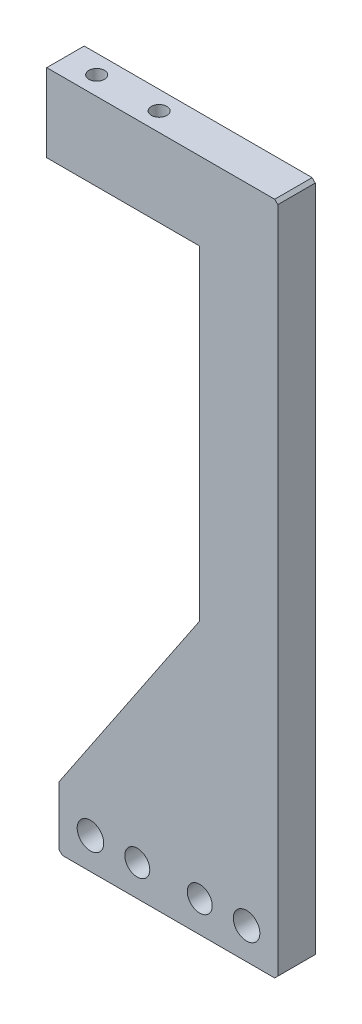
SolidWorks part; units mm, degrees
material "AISI 1045 钢，冷拔"
ref_plane "前视基准面" through (0, 0, 0) normal (0, 0, 1) x (1, 0, 0)
ref_plane "上视基准面" through (0, 0, 0) normal (0, 1, 0) x (1, 0, 0)
ref_plane "右视基准面" through (0, 0, 0) normal (1, 0, 0) x (0, 0, -1)
sketch "草图1" plane through (0, 0, 0) normal (0, 0, 1) x (1, 0, 0)
  line L0 (74.8691, -20) -> (4.8691, -20)
  line L1 (4.8691, -20) -> (4.8691, 0)
  line L3 (4.8691, 0) -> (49.8691, 67.0298)
  line L5 (49.8691, 67.0298) -> (49.8691, 171)
  line L6 (49.8691, 171) -> (0.8691, 171)
  line L7 (0.8691, 171) -> (0.8691, 196)
  line L8 (0.8691, 196) -> (74.8691, 196)
  line L9 (74.8691, 196) -> (74.8691, -20)
  dimension "D1" = 25
  dimension "D2" = 25
  dimension "D3" = 70
  dimension "D4" = 74
extrude "凸台-拉伸1" add sketch "草图1" against normal blind 12
hole_wizard "Ø8.5 (8.5) 直径孔1" positions "草图3" profile "草图4" hole size "Ø8.5" standard "Ansi Metric"
sketch "草图3" plane through (0, 0, 0) normal (0, 0, 1) x (1, 0, 0)
  line L0 (74.8691, -20) -> (74.8691, 196) construction
  line L1 (4.8691, -20) -> (74.8691, -20) construction
  point P0 (64.8691, -10)
  point P2 (14.8691, -10)
  dimension "D1" = 10
  dimension "D2" = 50
  dimension "D3" = 10
sketch "草图4" plane through (64.8691, -10, 0) normal (1, 0, 0) x (0, -1, 0)
  line L0 (0, 0) -> (0, 18.0637)
  line L1 (0, 18.0637) -> (4.25, 15.61)
  line L2 (4.25, 15.61) -> (4.25, 0)
  line L5 (4.25, 0) -> (0, 0)
  line L10 (0, 18.0637) -> (-4.25, 15.61) construction
  line L11 (0, -6.35) -> (0, 107.95) construction
  dimension "孔直径" = 8.5
  dimension "孔深度" = 15.61
  dimension "导头角度" = 120
sketch "草图5" plane through (0, 0, 0) normal (0, 0, 1) x (1, 0, 0)
  line L0 (4.8691, -20) -> (74.8691, -20) construction
  line L3 (74.8691, -20) -> (74.8691, 196) construction
  circle A0 centre (29.8691, -10) radius 4
  circle A1 centre (49.8691, -10) radius 4
  dimension "D1" = 8
  dimension "D3" = 8
  dimension "D2" = 10
  dimension "D4" = 25
  dimension "D5" = 20
extrude "切除-拉伸1" cut sketch "草图5" against normal blind 12
hole_wizard "M6 螺纹孔1" positions "草图7" profile "草图6" tap size "M6" standard "Iso"
sketch "草图7" plane through (0, 196, 0) normal (0, 1, 0) x (1, 0, 0)
  line L0 (0.8691, 12) -> (0.8691, 0) construction
  line L1 (74.8691, 12) -> (0.8691, 12) construction
  point P0 (10.8691, 6)
  point P2 (30.8691, 6)
  point P5 (0.8691, 6)
  dimension "D1" = 10
  dimension "D2" = 20
  dimension "D3" = 6
  dimension "D4" = 6
sketch "草图6" plane through (10.8691, 196, -6) normal (1, 0, 0) x (0, 0, 1)
  line L0 (0, 0) -> (0, 25)
  line L1 (0, 25) -> (2.5, 25)
  line L2 (2.5, 25) -> (2.5, 0)
  line L5 (2.5, 0) -> (0, 0)
  line L11 (0, -6.35) -> (0, 107.95) construction
  dimension "通孔螺纹孔钻头直径" = 5
  dimension "通孔螺纹孔钻头深度" = 25
cosmetic thread "孔螺蚊线1" parameters "D2"=6
cosmetic thread "孔螺蚊线2" parameters "D2"=6
chamfer "倒角1" distance 1 angle 45 2 edges at (74.8691, -20, -6) (74.8691, 196, -6)
chamfer "倒角2" distance 1 angle 45 1 edges at (4.8691, -20, -6)
